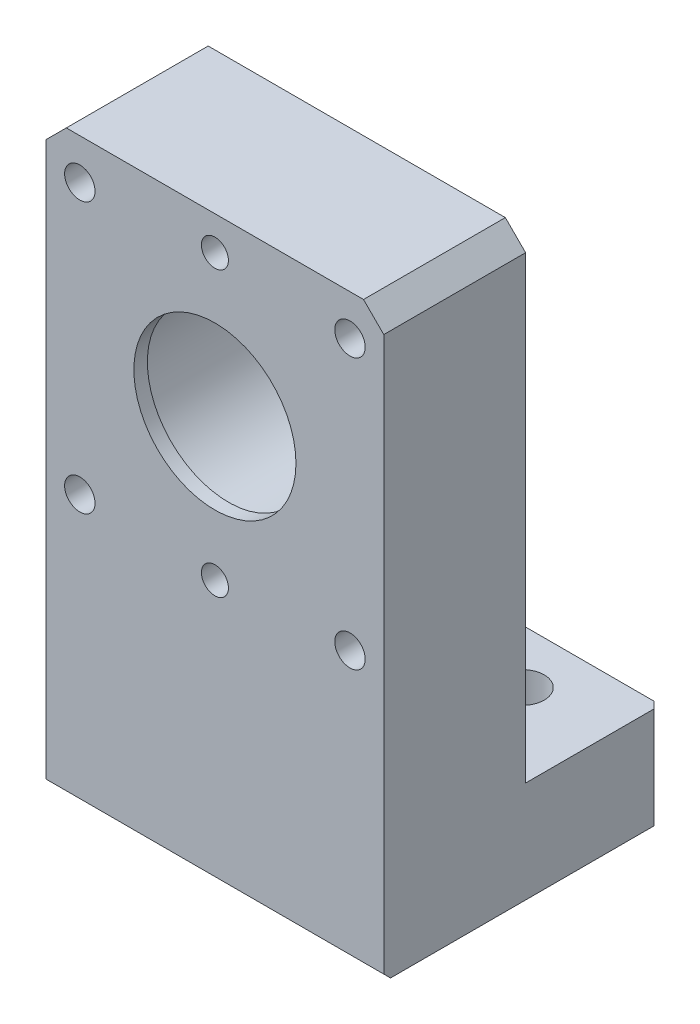
from build123d import *

# Parameters (mm, degrees)
SKETCH3_W                                            = 50
SKETCH3_H                                            = 86
SKETCH3_R                                            = 14
BOSS_EXTRUDE1_DEPTH                                  = 21
M3_TAPPED_HOLE1_D                                    = 2.5
M3_TAPPED_HOLE1_DEPTH                                = 10
M3_TAPPED_HOLE1_TIP                                  = 0.751075774
BOSS_EXTRUDE3_START                                  = -2
SKETCH4_R                                            = 14
SKETCH4_R_2                                          = 12
BOSS_EXTRUDE3_DEPTH                                  = 2
F_4_0_4_DIAMETER_HOLE2_D                             = 4
SKETCH22_W                                           = 50
SKETCH22_H                                           = 15
BOSS_EXTRUDE5_DEPTH                                  = 20
SKETCH23_R                                           = 3.25
CUT_EXTRUDE3_DEPTH                                   = 92.989129793
F_4_0_4_DIAMETER_HOLE1_D                             = 4
F_4_0_4_DIAMETER_HOLE1_DEPTH                         = 15
F_4_0_4_DIAMETER_HOLE1_TIP                           = 1.201721238
HOLE_SIZE_PER_SOCKET_HEAD_CAP_SCREW_TYPE_D           = 4.5
HOLE_SIZE_PER_SOCKET_HEAD_CAP_SCREW_TYPE_CBORE_D     = 8
HOLE_SIZE_PER_SOCKET_HEAD_CAP_SCREW_TYPE_CBORE_DEPTH = 4.6
CHAMFER1_SIZE                                        = 3
CHAMFER2_SIZE                                        = 1


with BuildPart() as part:
    # Sketch3 → Boss-Extrude1 (new body)
    with BuildSketch(Plane.XY):
        with Locations((0, 43)):
            Rectangle(SKETCH3_W, SKETCH3_H)
        with Locations(Location((0, 60, 0), (0, 0, 180))):
            Circle(SKETCH3_R, mode=Mode.SUBTRACT)
    extrude(amount=BOSS_EXTRUDE1_DEPTH)

    # M3 Tapped Hole1
    with Locations(Plane(origin=(6.398868237, 17.925711715, 0), x_dir=(1, 0, 0), z_dir=(0, 0, -1))):
        with Locations((11.601131763, -42.074288285), (-24.398868237, -42.074288285)):
            Hole(M3_TAPPED_HOLE1_D / 2, depth=M3_TAPPED_HOLE1_DEPTH)
            with Locations((0, 0, -(M3_TAPPED_HOLE1_DEPTH + M3_TAPPED_HOLE1_TIP / 2))):  # 118° drill point
                Cone(0, M3_TAPPED_HOLE1_D / 2, M3_TAPPED_HOLE1_TIP, mode=Mode.SUBTRACT)

    # Sketch4 → Boss-Extrude3 (add)
    with BuildSketch(Plane.XY.offset(21).offset(BOSS_EXTRUDE3_START)):
        with Locations(Location((0, 60, 0), (0, 0, 180))):
            Circle(SKETCH4_R)
        with Locations((0, 60)):
            Circle(SKETCH4_R_2, mode=Mode.SUBTRACT)
    extrude(amount=BOSS_EXTRUDE3_DEPTH)

    # Ø4.0 (4) Diameter Hole2 (through all)
    with Locations(Plane.XY.offset(21)):
        with Locations((0, 81), (0, 39)):
            Hole(F_4_0_4_DIAMETER_HOLE2_D / 2)

    # Sketch22 → Boss-Extrude5 (add)
    with BuildSketch(Plane(origin=(0, 0, 0), x_dir=(-1, 0, 0), z_dir=(0, 0, -1))):
        with Locations((0, 7.5)):
            Rectangle(SKETCH22_W, SKETCH22_H)
    extrude(amount=BOSS_EXTRUDE5_DEPTH)

    # Sketch23 → Cut-Extrude3 (cut, through all)
    with BuildSketch(Plane.XZ):
        with Locations((12.5, -12)):
            Circle(SKETCH23_R)
        with Locations((-12.5, -12)):
            Circle(SKETCH23_R)
    extrude(amount=-CUT_EXTRUDE3_DEPTH, mode=Mode.SUBTRACT)

    # Ø4.0 (4) Diameter Hole1
    with Locations(Plane.XZ):
        with Locations((0, -15), (0, -5)):
            Hole(F_4_0_4_DIAMETER_HOLE1_D / 2, depth=F_4_0_4_DIAMETER_HOLE1_DEPTH)
            with Locations((0, 0, -(F_4_0_4_DIAMETER_HOLE1_DEPTH + F_4_0_4_DIAMETER_HOLE1_TIP / 2))):  # 118° drill point
                Cone(0, F_4_0_4_DIAMETER_HOLE1_D / 2, F_4_0_4_DIAMETER_HOLE1_TIP, mode=Mode.SUBTRACT)

    # Hole size per socket head cap screw type 1 (through all)
    with Locations(Plane(origin=(0, 0, 0), x_dir=(-1, 0, 0), z_dir=(0, 0, -1))):
        with Locations((-20, 80), (-20, 40), (20, 40), (20, 80)):
            CounterBoreHole(HOLE_SIZE_PER_SOCKET_HEAD_CAP_SCREW_TYPE_D / 2, HOLE_SIZE_PER_SOCKET_HEAD_CAP_SCREW_TYPE_CBORE_D / 2, HOLE_SIZE_PER_SOCKET_HEAD_CAP_SCREW_TYPE_CBORE_DEPTH)

    # Chamfer1
    chamfer1_edges = [part.edges().sort_by_distance(p)[0] for p in [
        (-25, 86, 10.5),
        (25, 86, 10.5),
    ]]
    chamfer(chamfer1_edges, length=CHAMFER1_SIZE)

    # Chamfer2
    chamfer2_edges = [part.edges().sort_by_distance(p)[0] for p in [
        (0, 0, 21),
        (25, 7.5, -20),
        (-25, 7.5, -20),
    ]]
    chamfer(chamfer2_edges, length=CHAMFER2_SIZE)


solid = part.part
